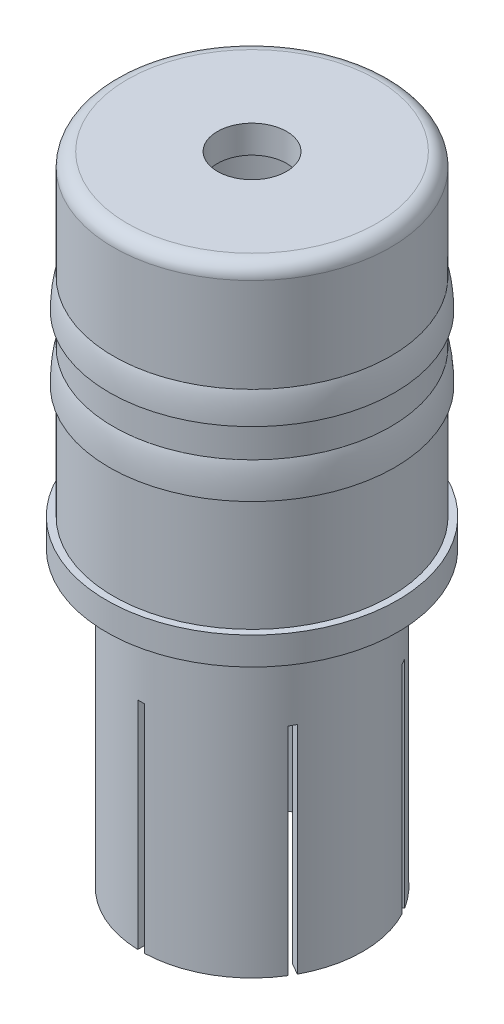
from build123d import *

# Parameters (mm, degrees)
FILLET1_R          = 0.5
SKETCH8_W          = 0.25
SKETCH8_H          = 8
CUT_EXTRUDE1_DEPTH = 6
CIRPATTERN1_COUNT  = 3


with BuildPart() as part:
    # Sketch1 → Revolve1 (revolve)
    with BuildSketch(Plane.XY, mode=Mode.PRIVATE) as revolve1_sk:
        with BuildLine():
            Line((-5, 3.1), (-5, -1))
            Line((-5, -1), (-5.25, -1))
            Line((-5.25, -1), (-5.25, -2))
            Line((-5.25, -2), (-4, -2))
            Line((-4, -2), (-4, -12.6))
            Line((-4, -12.6), (-3.5, -12.6))
            Line((-3.5, -12.6), (-3.5, 0))
            Line((-3.5, 0), (-3.125, 0))
            Line((-3.125, 0), (-3.125, 9.4))
            Line((-3.125, 9.4), (-1.25, 9.4))
            Line((-1.25, 9.4), (-1.25, 10.4))
            Line((-1.25, 10.4), (-5, 10.4))
            Line((-5, 10.4), (-5, 6.5))
            add(Edge.make_bspline(
                [(-5, 6.5), (-5.047605665, 6.363384357), (-5.0814919, 6.202637521), (-5.130093219, 5.840342723), (-5.144049999, 5.645135031), (-5.15, 5.440840859)],
                knots=[0, 0, 0, 0, 0.5, 0.5, 1, 1, 1, 1], degree=3))
            Line((-5.15, 5.440840859), (-5, 5.440840859))
            Line((-5, 5.440840859), (-5, 4.297032053))
            add(Edge.make_bspline(
                [(-5, 4.297032053), (-5.05121173, 4.142122175), (-5.086517142, 3.960249608), (-5.134772947, 3.550843087), (-5.146982855, 3.330472207), (-5.15, 3.1)],
                knots=[0, 0, 0, 0, 0.5, 0.5, 1, 1, 1, 1], degree=3))
            Line((-5.15, 3.1), (-5, 3.1))
        make_face()
    revolve(revolve1_sk.sketch.rotate(Axis((0, -30.576267402, 0), (0, 1, 0)), 270), axis=Axis((0, -30.576267402, 0), (0, 1, 0)))

    # Fillet1
    fillet1_edges = [part.edges().sort_by_distance(p)[0] for p in [
        (0, 10.4, 5),
    ]]
    fillet(fillet1_edges, radius=FILLET1_R)

    # Sketch8 → Cut-Extrude1 (cut, symmetric)
    with BuildSketch(Plane.XY):
        with Locations((0, -8.8)):
            Rectangle(SKETCH8_W, SKETCH8_H)
    cut_extrude1 = extrude(amount=CUT_EXTRUDE1_DEPTH, both=True, mode=Mode.SUBTRACT)

    # CirPattern1: Cut-Extrude1 ×3 about axis
    cirpattern1_axis = Axis((0, 0, 0), (0, 1, 0))
    for i in range(1, CIRPATTERN1_COUNT):
        add(cut_extrude1.rotate(cirpattern1_axis, i * 360 / CIRPATTERN1_COUNT), mode=Mode.SUBTRACT)


solid = part.part
